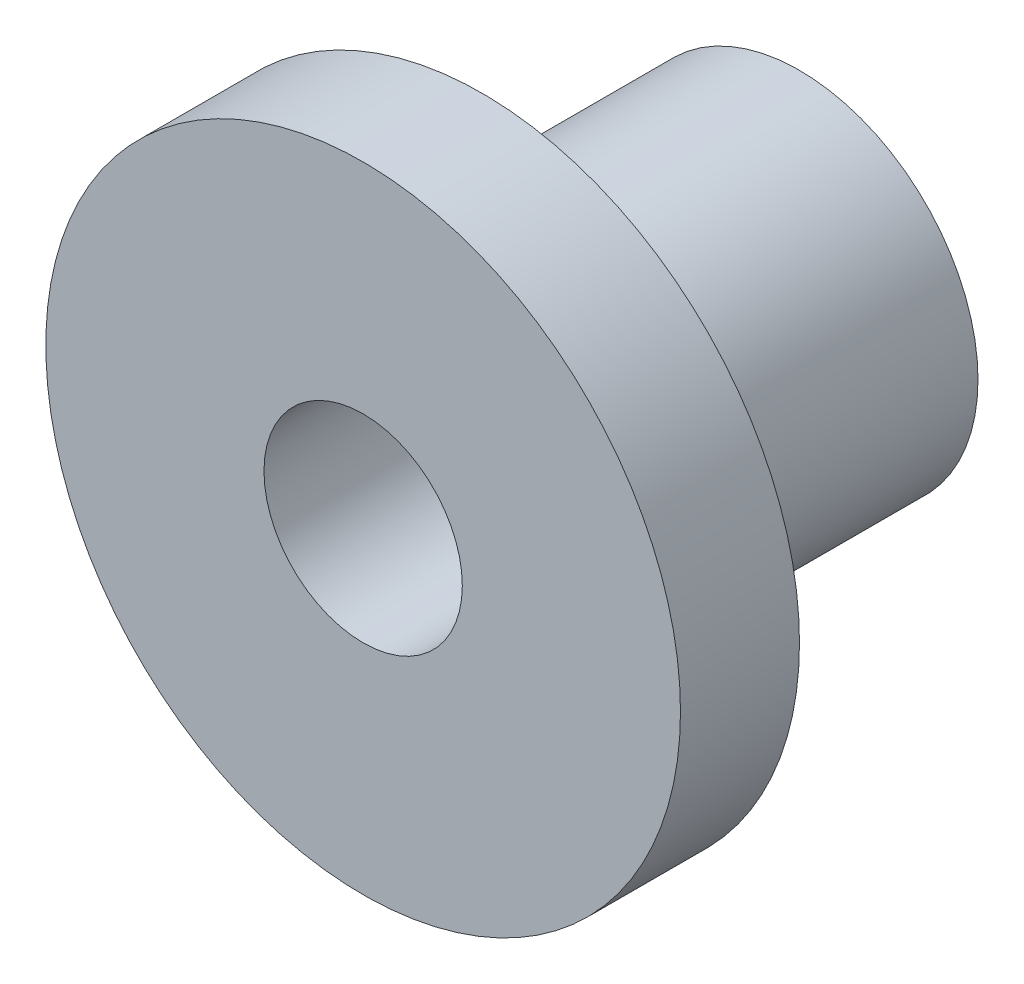
SolidWorks part; units mm, degrees
ref_plane "Front Plane" through (0, 0, 0) normal (0, 0, 1) x (1, 0, 0)
ref_plane "Top Plane" through (0, 0, 0) normal (0, 1, 0) x (1, 0, 0)
ref_plane "Right Plane" through (0, 0, 0) normal (1, 0, 0) x (0, 0, -1)
sketch "Sketch1" plane through (0, 0, 0) normal (0, 0, 1) x (1, 0, 0)
  circle A0 centre (0, 0) radius 22.5
  dimension "D1" = 45
extrude "Boss-Extrude1" add sketch "Sketch1" along normal blind 40
sketch "Sketch2" plane through (0, 0, 40) normal (0, 0, 1) x (1, 0, 0)
  circle A0 centre (0, 0) radius 40
  dimension "D1" = 80
extrude "Boss-Extrude2" add sketch "Sketch2" along normal blind 15
sketch "Sketch3" plane through (0, 0, 0) normal (0, 0, -1) x (-1, 0, 0)
  circle A0 centre (0, 0) radius 12.5
  dimension "D1" = 25
extrude "Cut-Extrude1" cut sketch "Sketch3" against normal blind 97
